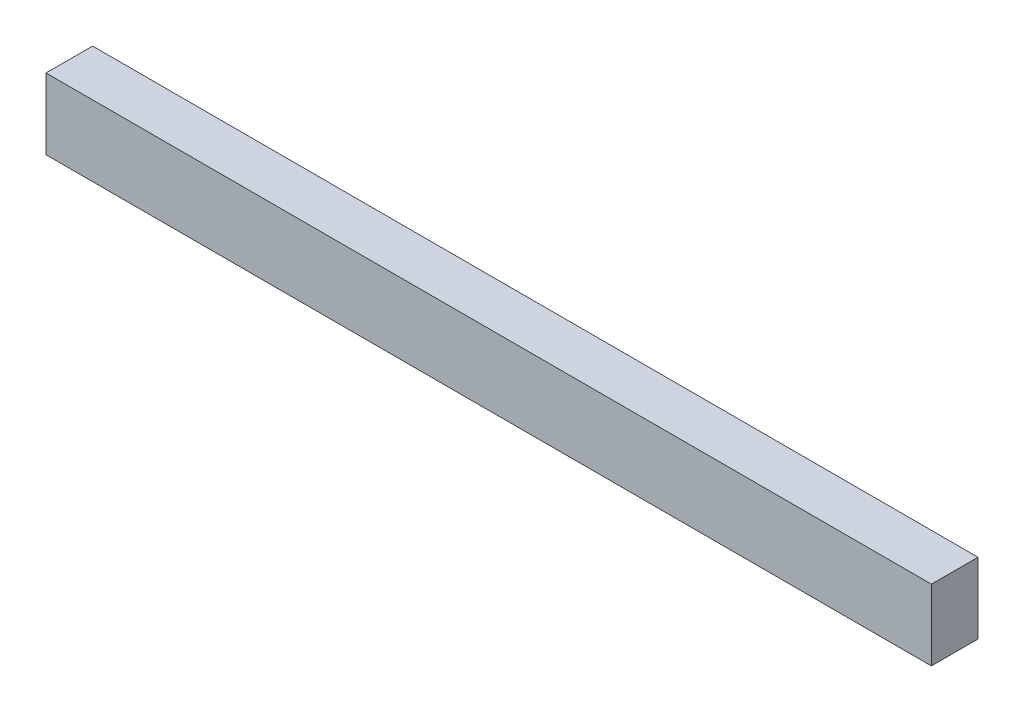
SolidWorks part; units mm, degrees
ref_plane "Front Plane" through (0, 0, 0) normal (0, 0, 1) x (1, 0, 0)
ref_plane "Top Plane" through (0, 0, 0) normal (0, 1, 0) x (1, 0, 0)
ref_plane "Right Plane" through (0, 0, 0) normal (1, 0, 0) x (0, 0, -1)
sketch "Sketch1" plane through (0, 0, 0) normal (0, 0, 1) x (1, 0, 0)
  line L1 (-237.5, 19) -> (237.5, 19)
  line L2 (-237.5, 19) -> (-237.5, -19)
  line L3 (-237.5, -19) -> (237.5, -19)
  line L4 (237.5, 19) -> (237.5, -19)
  line L5 (-237.5, 19) -> (237.5, -19) construction
  line L6 (-237.5, -19) -> (237.5, 19) construction
  point P0 (0, 0)
  dimension "D1" = 475
  dimension "D2" = 38
extrude "Boss-Extrude1" add sketch "Sketch1" along normal blind 25
